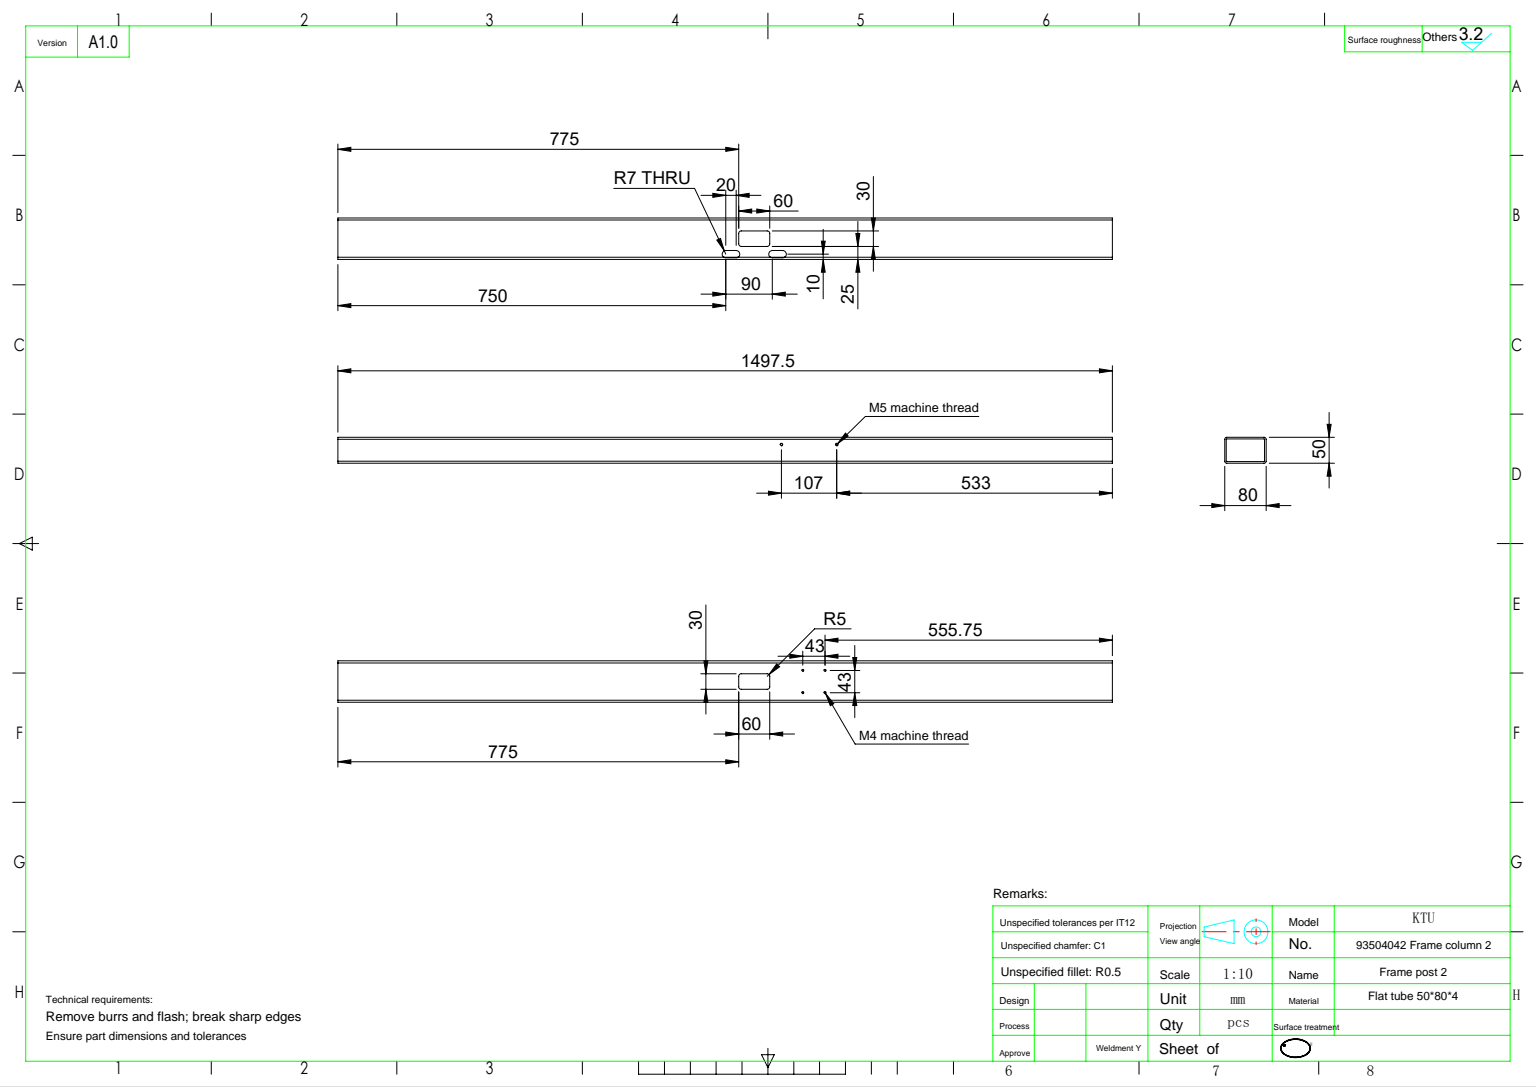
SolidWorks part; units mm, degrees
ref_plane "前视基准面" through (0, 0, 0) normal (0, 0, 1) x (1, 0, 0)
ref_plane "上视基准面" through (0, 0, 0) normal (0, 1, 0) x (1, 0, 0)
ref_plane "右视基准面" through (0, 0, 0) normal (1, 0, 0) x (0, 0, -1)
sketch "草图1" plane through (0, 0, 0) normal (0, 0, 1) x (1, 0, 0)
  line L1 (-36, 25) -> (36, 25)
  line L2 (-40, 21) -> (-40, -21)
  line L3 (-36, -25) -> (36, -25)
  line L4 (40, 21) -> (40, -21)
  line L5 (-40, 25) -> (40, -25) construction
  line L6 (-40, -25) -> (40, 25) construction
  arc A0 (36, -25) -> (40, -21) centre (36, -21) ccw
  arc A1 (-40, -21) -> (-36, -25) centre (-36, -21) ccw
  arc A2 (36, 25) -> (40, 21) centre (36, 21) cw
  arc A3 (-36, 25) -> (-40, 21) centre (-36, 21) ccw
  point P0 (0, 0)
  dimension "D3" = 4
  dimension "D1" = 50
  dimension "D2" = 80
extrude "拉伸-薄壁1" add sketch "草图1" along normal mid plane 1497.5 thin
sketch "草图4" plane through (0, -25, 0) normal (0, -1, 0) x (1, 0, 0)
  line L0 (30, 91.25) -> (30, 111.25) construction
  line L1 (23, 91.25) -> (23, 111.25)
  line L2 (37, 91.25) -> (37, 111.25)
  line L3 (30, 1.25) -> (30, 21.25) construction
  line L4 (23, 1.25) -> (23, 21.25)
  line L5 (37, 1.25) -> (37, 21.25)
  arc A0 (23, 91.25) -> (37, 91.25) centre (30, 91.25) ccw
  arc A1 (37, 111.25) -> (23, 111.25) centre (30, 111.25) ccw
  arc A2 (23, 1.25) -> (37, 1.25) centre (30, 1.25) ccw
  arc A3 (37, 21.25) -> (23, 21.25) centre (30, 21.25) ccw
  point P2 (30, 101.25)
  point P9 (30, 11.25)
  dimension "D1" = 7
  dimension "D2" = 20
extrude "切除-拉伸2" cut sketch "草图4" against normal blind 10
sketch "草图5" plane through (0, -25, 0) normal (0, -1, 0) x (1, 0, 0)
  line L0 (30, 91.25) -> (30, 21.25) construction
  line L1 (30, 56.25) -> (-56.5957, 56.25) construction
  line L2 (40, 748.75) -> (40, -748.75) construction
  line L3 (-10, 26.25) -> (10, 26.25)
  line L4 (-15, 31.25) -> (-15, 81.25)
  line L5 (-10, 86.25) -> (10, 86.25)
  line L6 (15, 31.25) -> (15, 81.25)
  line L7 (-15, 26.25) -> (15, 86.25) construction
  line L8 (-15, 86.25) -> (15, 26.25) construction
  arc A0 (-10, 26.25) -> (-15, 31.25) centre (-10, 31.25) cw
  arc A1 (10, 26.25) -> (15, 31.25) centre (10, 31.25) ccw
  arc A2 (10, 86.25) -> (15, 81.25) centre (10, 81.25) cw
  arc A3 (-15, 81.25) -> (-10, 86.25) centre (-10, 81.25) cw
  point P6 (0, 56.25)
  dimension "D4" = 5
  dimension "D1" = 30
  dimension "D2" = 60
  dimension "D3" = 40
extrude "切除-拉伸3" cut sketch "草图5" against normal through all
sketch "草图6" plane through (0, 25, 0) normal (0, 1, 0) x (1, 0, 0)
  line L0 (-40, -748.75) -> (-40, 748.75) construction
  circle A0 centre (-21.5, -150) radius 1.65
  circle A1 centre (-21.5, -193) radius 1.65
  circle A2 centre (21.5, -150) radius 1.65
  circle A3 centre (21.5, -193) radius 1.65
  dimension "D1" = 3.3
  dimension "D2" = 43
  dimension "D3" = 43
  dimension "D4" = 150
  dimension "D5" = 18.5
extrude "切除-拉伸4" cut sketch "草图6" against normal blind 10
cosmetic thread "装饰螺纹线1" parameters "D2"=4
cosmetic thread "装饰螺纹线2" parameters "D2"=4
cosmetic thread "装饰螺纹线3" parameters "D2"=4
cosmetic thread "装饰螺纹线4" parameters "D2"=4
sketch "草图7" plane through (-40, 0, 0) normal (-1, 0, 0) x (0, 0, 1)
  line L1 (748.75, 25) -> (-748.75, 25) construction
  line L2 (748.75, 21) -> (748.75, -21) construction
  circle A0 centre (108.75, 11) radius 2.1
  circle A1 centre (215.75, 11) radius 2.1
  dimension "D1" = 4.2
  dimension "D2" = 107
  dimension "D4" = 533
  dimension "D3" = 14
extrude "切除-拉伸5" cut sketch "草图7" against normal blind 10
cosmetic thread "装饰螺纹线5" parameters "D2"=5
cosmetic thread "装饰螺纹线6" parameters "D2"=5
